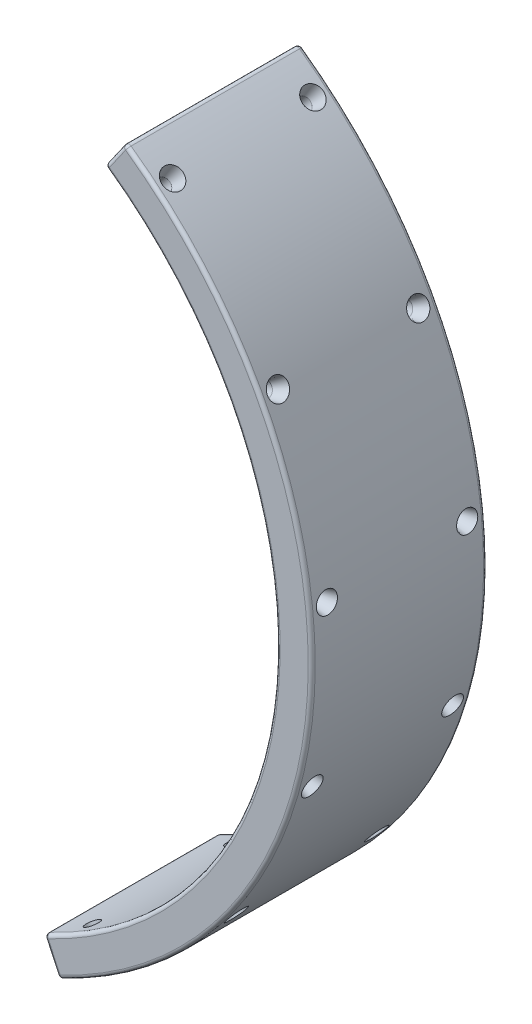
SolidWorks part; units mm, degrees
ref_plane "Front" through (0, 0, 0) normal (0, 0, 1) x (1, 0, 0)
ref_plane "Top" through (0, 0, 0) normal (0, 1, 0) x (1, 0, 0)
ref_plane "Right" through (0, 0, 0) normal (1, 0, 0) x (0, 0, -1)
sketch "Sketch1" plane through (0, 0, 0) normal (0, 0, 1) x (1, 0, 0)
  line L0 (0, 154.5871) -> (0, -145.8852) construction
  line L1 (143.3941, 204.788) -> (131.9226, 188.405)
  line L2 (105.6546, -226.5769) -> (97.2022, -208.4508)
  line L3 (0, 0) -> (89.7848, 128.226) construction
  line L4 (0, 0) -> (63.4796, -136.1325) construction
  line L5 (-151.8415, 0) -> (384.3455, 0) construction
  arc A0 (97.2022, -208.4508) -> (131.9226, 188.405) centre (0, 0) ccw
  arc A1 (105.6546, -226.5769) -> (143.3941, 204.788) centre (0, 0) ccw
  dimension "D1" = 460
  dimension "D2" = 500
  dimension "D6" = 523.5988
  dimension "D4" = 35
  dimension "D5" = 25
extrude "Extrude1" add sketch "Sketch1" along normal mid plane 100
fillet "Fillet1" radius 2 12 edges at (101.4284, -217.5139, 50) (101.4284, -217.5139, -50) (137.6583, 196.5965, 50) (137.6583, 196.5965, -50) (105.6546, -226.5769, 0) (97.2022, -208.4508, 0) (131.9226, 188.405, 0) (143.3941, 204.788, 0) (229.1248, -20.0458, -50) (249.0487, -21.7889, -50) (229.1248, -20.0458, 50) (249.0487, -21.7889, 50)
ref_plane "Plane1" through (0, 0, 40) normal (0, 0, 1) x (1, 0, 0)
sketch "Sketch2" plane through (0, 0, 40) normal (0, 0, 1) x (1, 0, 0)
  line L0 (-53.7263, 0) -> (397.788, 0) construction
  line L1 (0, 0) -> (212.1207, 252.7956) construction
  line L2 (143.1946, 179.987) -> (156.1006, 195.3678) construction
  line L3 (156.1006, 195.3678) -> (165.2932, 187.6544) construction
  line L4 (165.2932, 187.6544) -> (152.3871, 172.2735) construction
  line L5 (152.3871, 172.2735) -> (143.1946, 179.987) construction
  line L6 (152.3871, 172.2735) -> (147.7908, 176.1303) construction
  line L7 (147.7908, 176.1303) -> (155.1829, 184.9398) construction
  line L9 (165.2932, 187.6544) -> (160.6969, 191.5111)
  line L10 (160.6969, 191.5111) -> (155.1829, 184.9398)
  line L11 (155.1829, 184.9398) -> (158.2471, 182.3686)
  line L12 (158.2471, 182.3686) -> (165.2932, 187.6544)
  arc A0 (98.9956, -207.6051) -> (133.5419, 187.2607) centre (0, 0) ccw construction
  arc A1 (107.4784, -225.7175) -> (145.041, 203.6249) centre (0, 0) ccw construction
  dimension "D1" = 50
  dimension "D2" = 4
  dimension "D3" = 6
  dimension "D4" = 11.5
revolve "Cut-Revolve2" cut sketch "Sketch2" angle 360 about L10
sketch "Sketch3" plane through (155.1829, 184.9398, 0) normal (0.6428, 0.766, 0) x (0.766, -0.6428, 0)
  circle A0 centre (0, -40) radius 4 construction
  circle A1 centre (0, -40) radius 4
extrude "Cut-Extrude1" cut sketch "Sketch3" against normal up to next
ref_axis "Axis1" through (0, 0, 48) along (0, 0, -1)
pattern_circular "CirPattern1" count 6 over 110 about axis through (0, 0, 48) along (0, 0, -1) of "Cut-Extrude1", "Cut-Revolve2"
mirror "Mirror1" about plane through (0, 0, 0) normal (0, 0, 1) of "Cut-Revolve2", "Cut-Extrude1", "CirPattern1"
